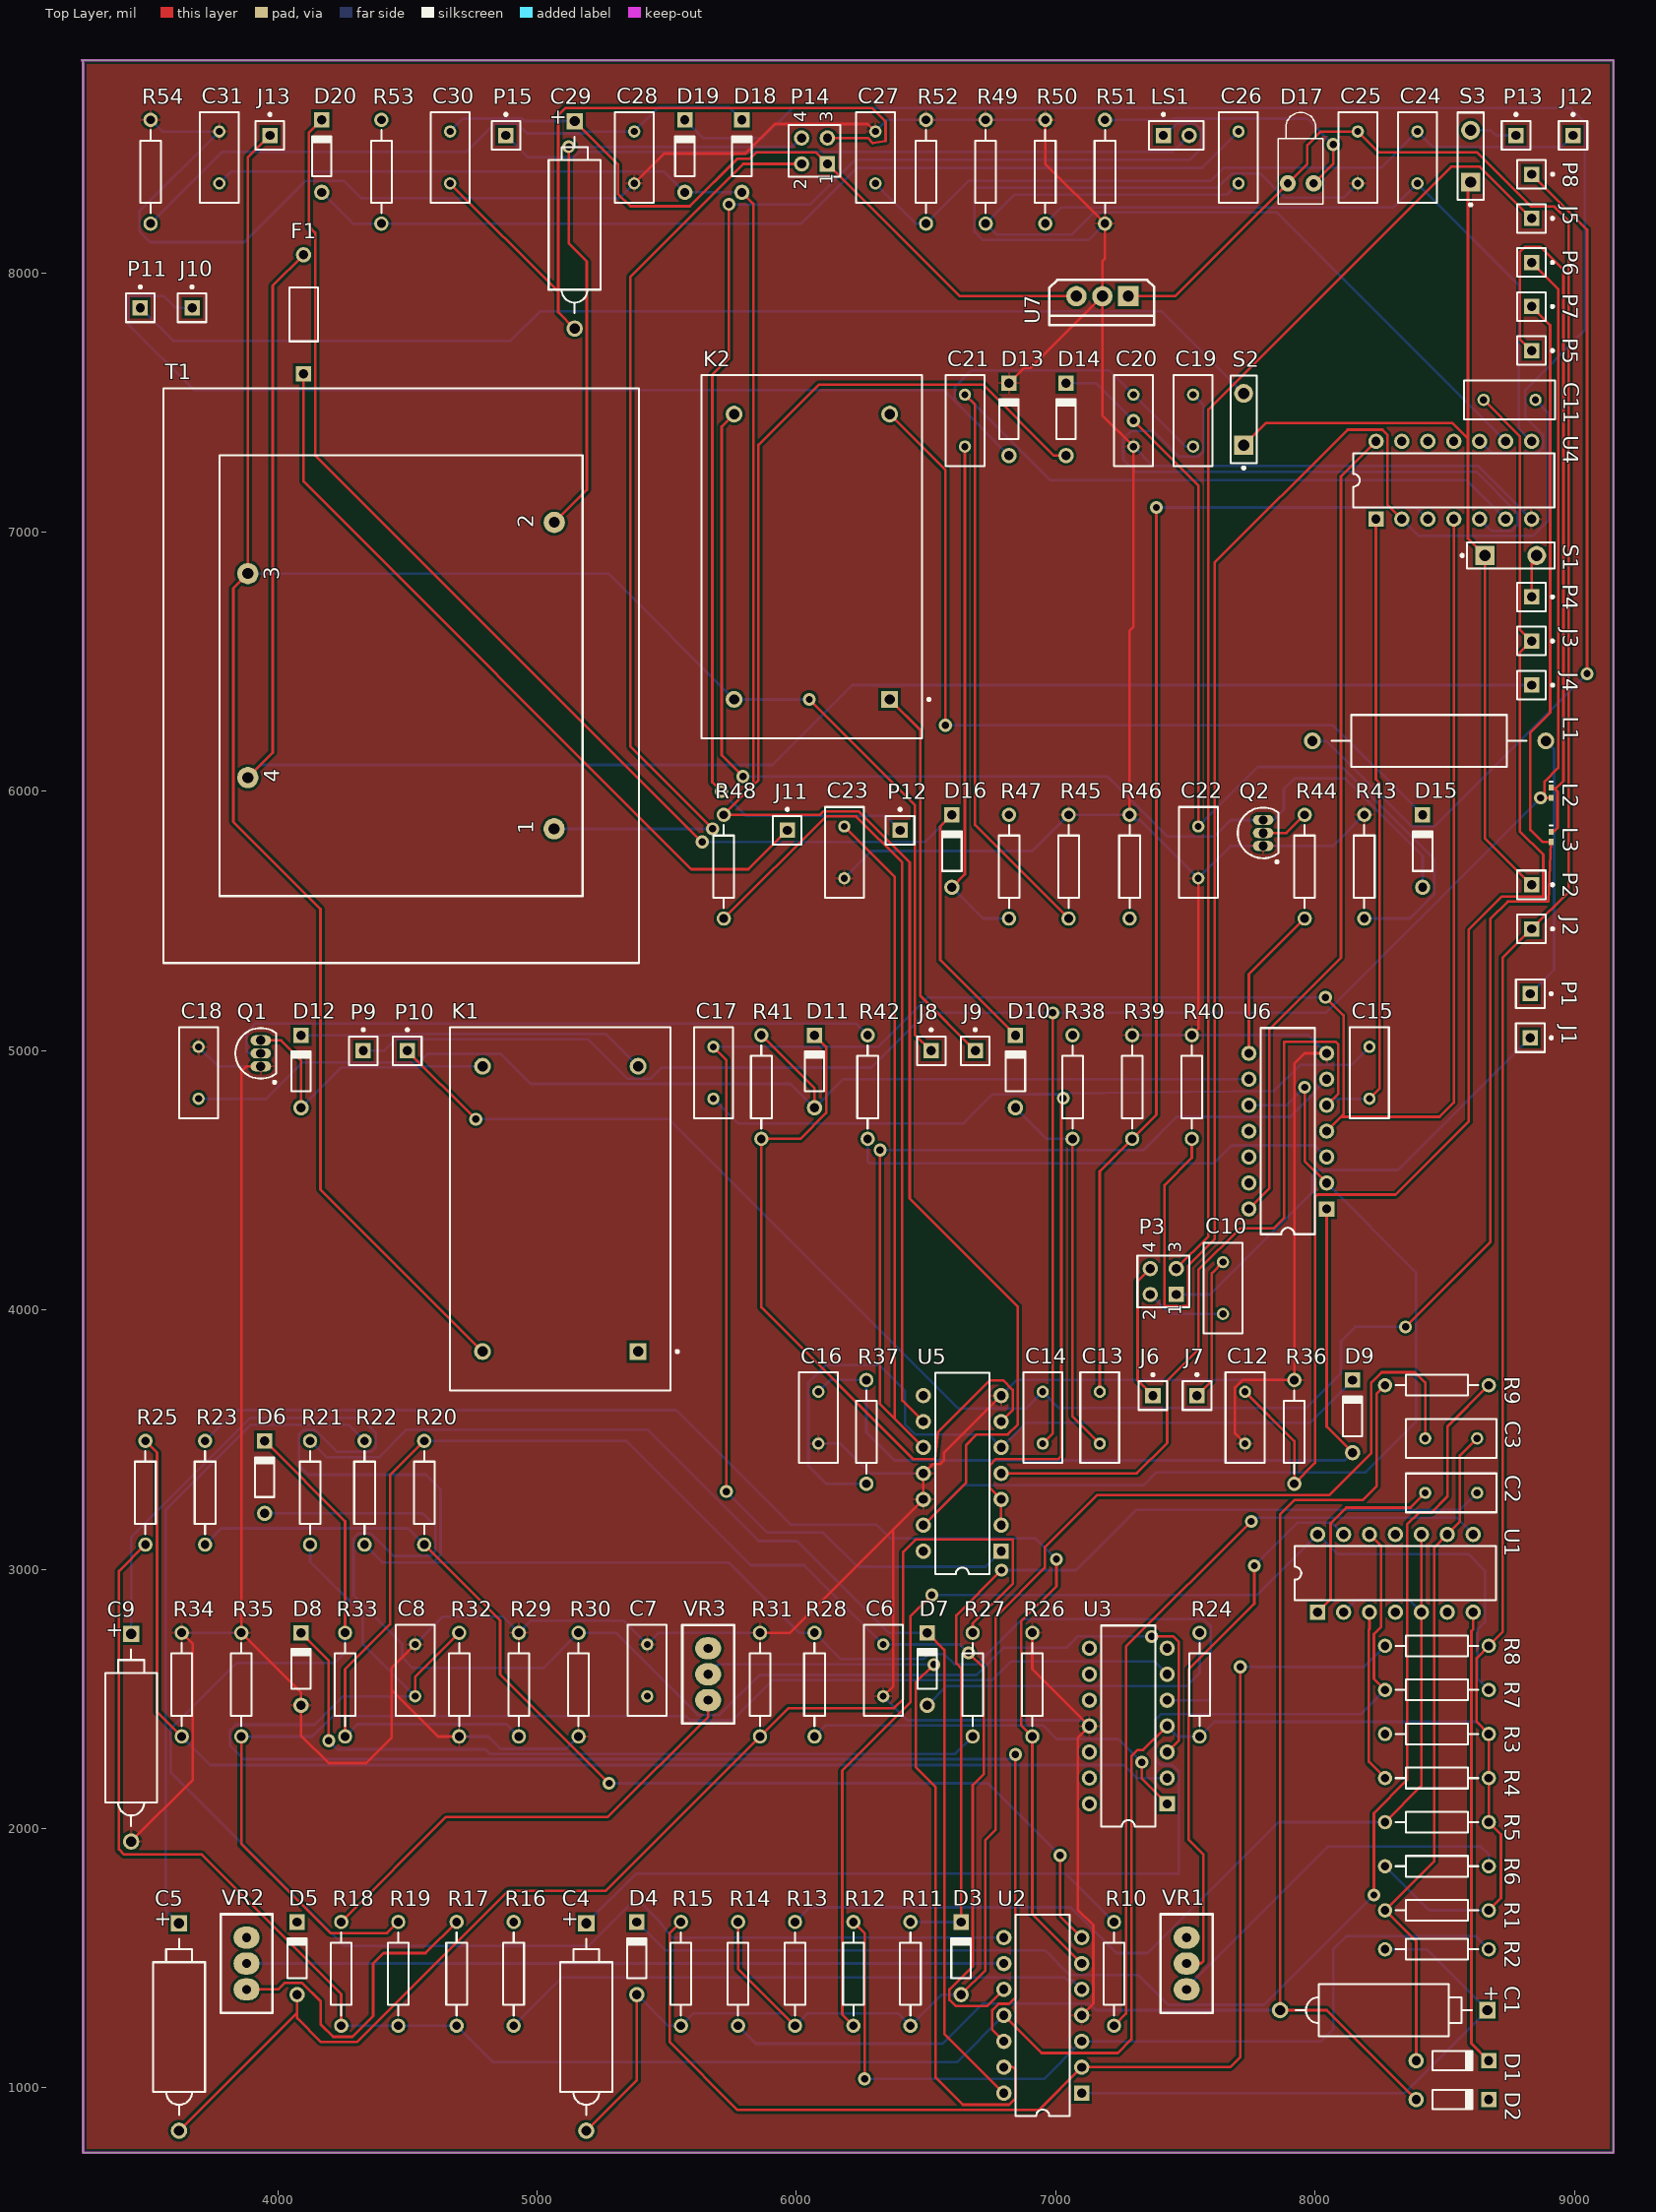
[diagram p0: Top Layer view]
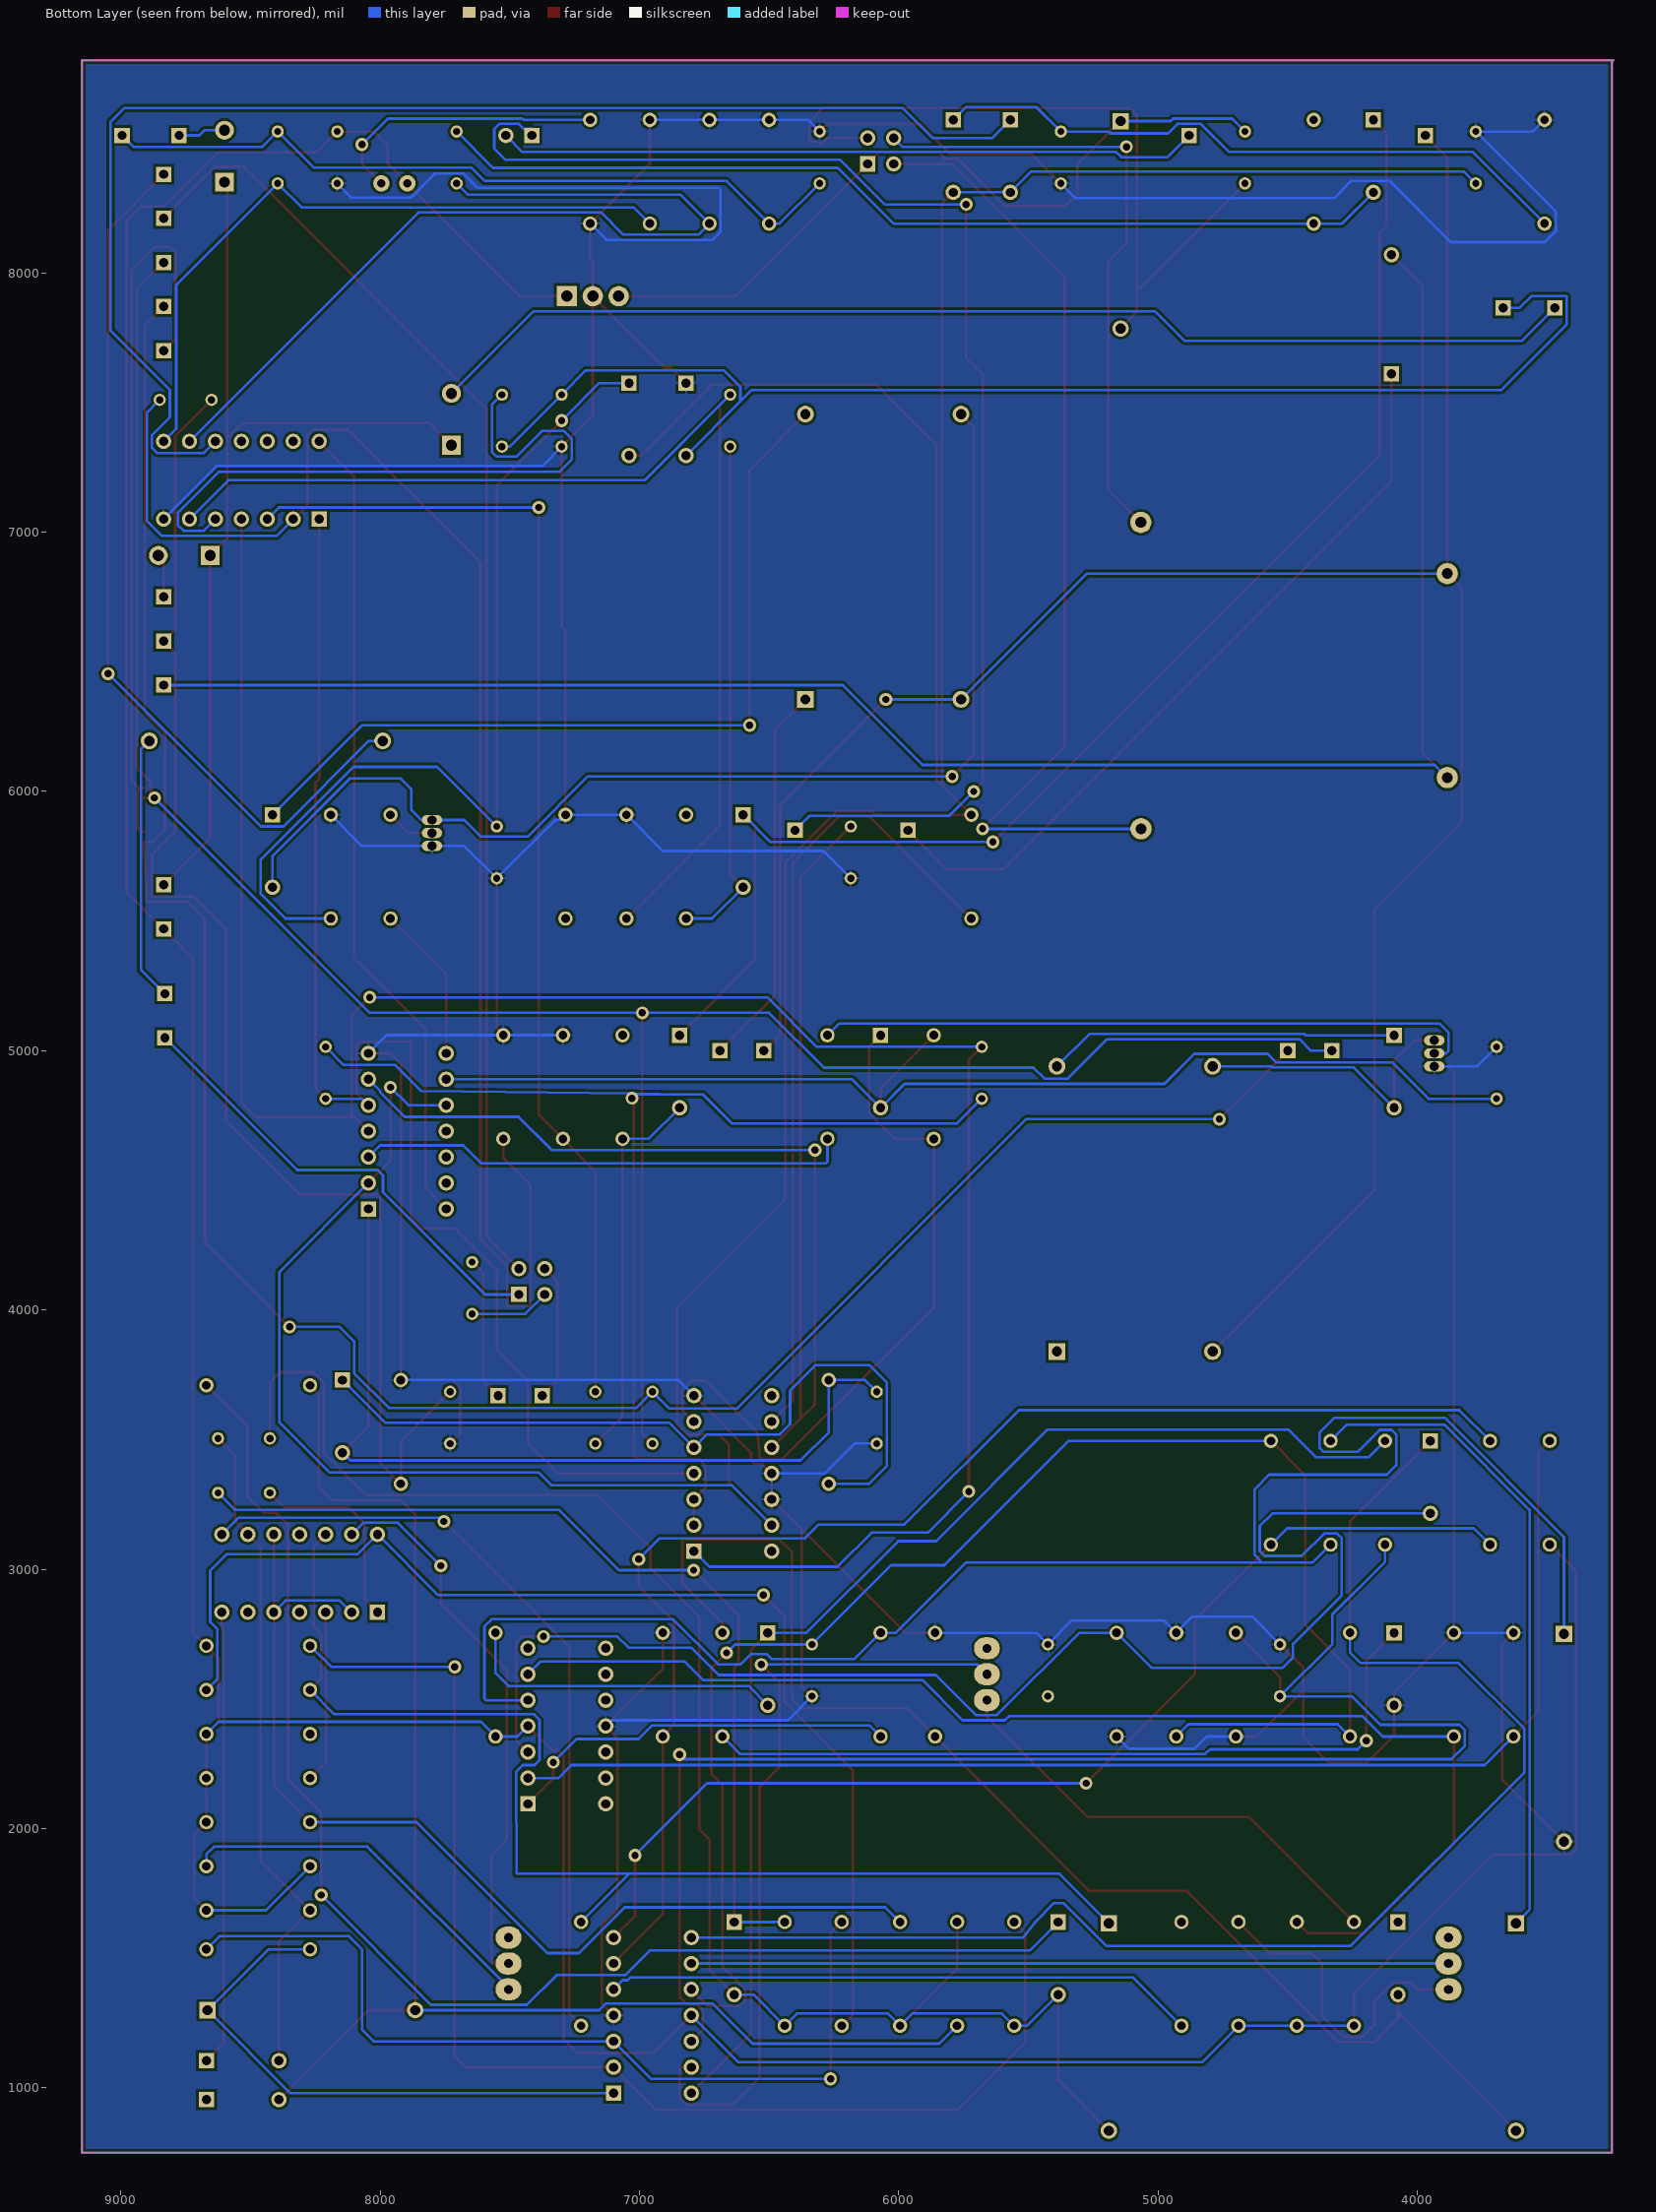
[diagram p1: Bottom Layer view, seen from below]
# Altium PCB MISC82089.PcbDoc (part 1 of 2)
Units mil, origin at the board's own origin, x right, y up, seen from the top; angles counter-clockwise.
Board outline 5905 x 8070 mil, 2 copper layers (Top Layer, Bottom Layer); 156 components, 100 nets, 374 pads, 37 vias.

## Layer stack, top to bottom (the 12.6 mil dielectric is the usual default, probably not edited)
Top Solder: solder mask 0.4, Solder Resist, Dk 3.5
Top Layer: signal copper 1.4
Dielectric 1: dielectric 12.6, FR-4, Dk 4.8
Bottom Layer: signal copper 1.4
Bottom Solder: solder mask 0.4, Solder Resist, Dk 3.5

## Board outline
3250,8750 3250,8807.93 ccw(c3232.93,8807.93) 3245,8820 9150,8820 9150,750 3250,750

## Design rules (kind name [scope] priority, off if disabled: settings)
Clearance [All] p1: gap=10
MinimumSolderMaskSliver [All] p1: minsoldermaskwidth=0
PolygonConnect [All] p1: connectstyle=Relief reliefconductorwidth=10 reliefentries=4 polygonreliefangle="90 Angle" airgapwidth=10
RoutingVias [All] p1: holewidth=28 width=50 viastyle="Through Hole" minholewidth=28 minwidth=50 maxholewidth=28 maxwidth=50
SilkToSilkClearance [All] p1: silktosilkclearance=0
SilkToSolderMaskClearance [IsPad] p1: minsilkscreentomaskgap=0 clearancetoexposedcopper=TRUE
SolderMaskExpansion [All] p1: expansion=4
Width [All] p1: maxlimit=10 minlimit=10 preferedwidth=10
27 further rules are at their usual default settings.

## Components (designator, comment, footprint, x,y, rotation, side; value= is the part's Value field where it differs from the comment)
C1 "220UF" POLAR0.8 8265,1300 r0 top
C2 "0.002" RAD-0.2 8525,3295 r0 top
C3 "104" RAD-0.2 8525,3505 r0 top
C4 "220UF" POLAR0.8 5190,1235 r90 top
C5 "10U" POLAR0.8 3620,1235 r90 top
C6 "104" RAD-0.2 6335,2610.5 r90 top
C7 "105" RAD-0.2 5425,2610.5 r90 top
C8 "105" RAD-0.2 4530,2610.5 r90 top
C9 "220UF" POLAR0.8 3435,2350.5 r90 top
C10 "3.3U" RAD-0.2 7645,4085 r90 top
C11 "105" RAD-0.2 8750,7510 r0 top
C12 "105" RAD-0.2 7730,3585 r90 top
C13 "105" RAD-0.2 7170,3585 r90 top
C14 "3.3U" RAD-0.2 6950,3585 r90 top
C15 "104" RAD-0.2 8210,4915 r90 top
C16 "3.3U" RAD-0.2 6085,3585 r90 top
C17 "104" RAD-0.2 5680,4915 r90 top
C18 "3.3U" RAD-0.2 3695,4915 r90 top
C19 "104" RAD-0.2 7530,7430 r90 top
C20 "104" RAD-0.2 7300,7430 r90 top
C21 "104" RAD-0.2 6650,7430 r90 top
C22 "105" RAD-0.2 7550,5765 r90 top
C23 "104" RAD-0.2 6185,5765 r90 top
C24 "105" RAD-0.2 8395,8445 r90 top
C25 "105" RAD-0.2 8165,8445 r90 top
C26 "105" RAD-0.2 7705,8445 r90 top
C27 "105" RAD-0.2 6305,8445 r90 top
C28 "105" RAD-0.2 5375,8445 r90 top
C29 "220UF" POLAR0.8 5145,8185 r90 top
C30 "105" RAD-0.2 4665,8445 r90 top
C31 "105" RAD-0.2 3775,8445 r90 top
D1 "4148" DO-35 8530,1105 r0 top
D2 "4148" DO-35 8530,955 r0 top
D3 "4148" DO-35 6635,1500 r90 top
D4 "4148" DO-35 5385,1500 r90 top
D5 "4148" DO-35 4075,1500 r90 top
D6 "4148" DO-35 3950,3355.5 r90 top
D7 "4148" DO-35 6505,2615.5 r90 top
D8 "4148" DO-35 4090,2615.5 r90 top
D9 "4148" DO-35 8145,3590 r90 top
D10 "4148" DO-35 6845,4920 r90 top
D11 "4148" DO-35 6070,4920 r90 top
D12 "4148" DO-35 4090,4920 r90 top
D13 "4148" DO-35 6820,7435 r90 top
D14 "4148" DO-35 7040,7435 r90 top
D15 "4148" DO-35 8415,5770 r90 top
D16 "4148" DO-35 6600,5770 r90 top
D17 "LED1" LED-1 7945,8345 r90 top
D18 "4148" DO-35 5790,8450 r90 top
D19 "4148" DO-35 5570,8450 r90 top
D20 "4148" DO-35 4170,8450 r90 top
F1 "Fuse 1" PIN-W2/E2.8 4100,7840 r90 top
J1 "Socket" PIN1 8830,5050 r270 top
J2 "Socket" PIN1 8835,5470 r270 top
J3 "Socket" PIN1 8835,6580 r270 top
J4 "Socket" PIN1 8835,6410 r270 top
J5 "Socket" PIN1 8835,8210 r270 top
J6 "Socket" PIN1 7375,3670 r0 top
J7 "Socket" PIN1 7545,3670 r0 top
J8 "Socket" PIN1 6520,5000 r0 top
J9 "Socket" PIN1 6690,5000 r0 top
J10 "Socket" PIN1 3670,7865 r0 top
J11 "Socket" PIN1 5965,5850 r0 top
J12 "Socket" PIN1 8995,8530 r0 top
J13 "Socket" PIN1 3970,8530 r0 top
K1 "Relay-SPST" MODULE4 5090,4390 r90 top
K2 "Relay-SPST" MODULE4 6060,6905 r90 top
L1 "Inductor Iron" AXIAL-0.9 8440,6195 r0 top
L2 "Inductor" 0402-A 8910,5995 r270 top
L3 "Inductor" 0402-A 8910,5825 r270 top
LS1 "Bell" PIN2 7415,8530 r0 top
P1 "Plug" PIN1 8830,5220 r270 top
P2 "Plug" PIN1 8835,5640 r270 top
P3 "Header 2X2" HDR2X2 7465,4060 r90 top
P4 "Plug" PIN1 8835,6750 r270 top
P5 "Plug" PIN1 8835,7700 r270 top
P6 "Plug" PIN1 8835,8040 r270 top
P7 "Plug" PIN1 8835,7870 r270 top
P8 "Plug" PIN1 8835,8380 r270 top
P9 "Plug" PIN1 4330,5000 r0 top
P10 "Plug" PIN1 4500,5000 r0 top
P11 "Plug" PIN1 3470,7865 r0 top
P12 "Plug" PIN1 6400,5850 r0 top
P13 "Plug" PIN1 8775,8530 r0 top
P14 "Header 2X2" HDR2X2 6120,8420 r90 top
P15 "Plug" PIN1 4880,8530 r0 top
Q1 "2N3904" TO-92A 3935,4990 r0 top
Q2 "2N3904" TO-92A 7800,5840 r0 top
R1 "17" AXIAL-0.4 8470,1685 r0 top
R2 "4" AXIAL-0.4 8470,1535 r0 top
R3 "8" AXIAL-0.4 8470,2365 r0 top
R4 "9" AXIAL-0.4 8470,2195 r0 top
R5 "10" AXIAL-0.4 8470,2025 r0 top
R6 "50" AXIAL-0.4 8470,1855 r0 top
R7 "50" AXIAL-0.4 8470,2535 r0 top
R8 "50" AXIAL-0.4 8470,2705 r0 top
R9 "24" AXIAL-0.4 8470,3710 r0 top
R10 "1.5K" AXIAL-0.4 7225,1440 r90 top
R11 "12" AXIAL-0.4 6440,1440 r90 top
R12 "22" AXIAL-0.4 6220,1440 r90 top
R13 "11" AXIAL-0.4 5995,1440 r90 top
R14 "2" AXIAL-0.4 5775,1440 r90 top
R15 "50" AXIAL-0.4 5555,1440 r90 top
R16 "20K" AXIAL-0.4 4910,1440 r90 top
R17 "50" AXIAL-0.4 4690,1440 r90 top
R18 "10K" AXIAL-0.4 4245,1440 r90 top
R19 "10K" AXIAL-0.4 4465,1440 r90 top
R20 "51" AXIAL-0.4 4565,3295.5 r90 top
R21 "330K" AXIAL-0.4 4125,3295.5 r90 top
R22 "10K" AXIAL-0.4 4335,3295.5 r90 top
R23 "50" AXIAL-0.4 3720,3295.5 r90 top
R24 "10K" AXIAL-0.4 7555,2555.5 r90 top
R25 "10K" AXIAL-0.4 3490,3295.5 r90 top
R26 "49" AXIAL-0.4 6910,2555.5 r90 top
R27 "1K" AXIAL-0.4 6680,2555.5 r90 top
R28 "1K" AXIAL-0.4 6070,2555.5 r90 top
R29 "35" AXIAL-0.4 4930,2555.5 r90 top
R30 "100K" AXIAL-0.4 5160,2555.5 r90 top
R31 "25K" AXIAL-0.4 5860,2555.5 r90 top
R32 "10K" AXIAL-0.4 4700,2555.5 r90 top
R33 "28" AXIAL-0.4 4260,2555.5 r90 top
R34 "3M" AXIAL-0.4 3630,2555.5 r90 top
R35 "10K" AXIAL-0.4 3860,2555.5 r90 top
R36 "49" AXIAL-0.4 7920,3530 r90 top
R37 "510K" AXIAL-0.4 6270,3530 r90 top
R38 "5.1K" AXIAL-0.4 7065,4860 r90 top
R39 "5.1K" AXIAL-0.4 7295,4860 r90 top
R40 "5.1K" AXIAL-0.4 7525,4860 r90 top
R41 "510K" AXIAL-0.4 5865,4860 r90 top
R42 "1K" AXIAL-0.4 6275,4860 r90 top
R43 "51K" AXIAL-0.4 8190,5710 r90 top
R44 "1K" AXIAL-0.4 7960,5710 r90 top
R45 "5.1K" AXIAL-0.4 7050,5710 r90 top
R46 "5.1K" AXIAL-0.4 7285,5710 r90 top
R47 "5.1K" AXIAL-0.4 6820,5710 r90 top
R48 "10K" AXIAL-0.4 5720,5710 r90 top
R49 "51K" AXIAL-0.4 6730,8390 r90 top
R50 "51K" AXIAL-0.4 6960,8390 r90 top
R51 "15K" AXIAL-0.4 7190,8390 r90 top
R52 "51K" AXIAL-0.4 6500,8390 r90 top
R53 "51K" AXIAL-0.4 4400,8390 r90 top
R54 "51K" AXIAL-0.4 3510,8390 r90 top
S1 "SW-PB" SPST-2 8755,6910 r0 top
S2 "SW-PB" SPST-2 7725,7435 r90 top
S3 "SW-PB" SPST-2 8600,8450 r90 top
T1 "Trans Eq" TRF_4 4475.83,6446.67 r90 top
U1 "LM324N" 646-06 8310,2985 r0 top
U2 "LM324N" 646-06 6950,1280 r90 top
U3 "LM324N" 646-06 7280,2395.5 r90 top
U4 "SN74LS02N" N014 8535,7200 r0 top
U5 "SN74LS74AN" 646-06 6640,3370 r90 top
U6 "SN74LS08J" J014 7895,4690 r90 top
U7 "LM7805" TO220A 7180,7910 r180 top
VR1 "10K" 3296W 7505,1480 r90 top
VR2 "10K" 3296W 3880,1480 r90 top
VR3 "10K" 3296W 5660,2595.5 r90 top

## Footprints (in the part's own frame and the unit in brackets; to place one, negate y for a bottom-side part, rotate by r counter-clockwise, add the part's x,y. Pads: shape width x height; smd on the part's side, far side on the other; paste and mask are expansions set on the pad)
0402-A [mm] "Chip Inductor, Body 1.0x0.5mm, IPC High Density"
  rect 0.6x0.5 smd: 1(-0.5,0) 2(0.5,0)
  silkscreen extent -1.1,-0.15 -1.1,0.15, body extent -0.55,-0.3 0.55,0.3, height 0.55
646-06 [mm] "DIP; 14 Leads; Row Spacing 7.62 mm; Pitch 2.54 mm"
  rect 1.5x1.5 hole 0.9: 1(-7.62,-3.81)
  round 1.5 hole 0.9: 2(-5.08,-3.81) 3(-2.54,-3.81) 4(0,-3.81) 5(2.54,-3.81) 6(5.08,-3.81) 7(7.62,-3.81) 8(7.62,3.81) 9(5.08,3.81) 10(2.54,3.81) 11(0,3.81) 12(-2.54,3.81) 13(-5.08,3.81) 14(-7.62,3.81)
  silkscreen extent -9.85,-2.65 9.85,2.65
3296W [mil]
  oval 85x100 hole 35: 1(-100,0) 2(0,0) 3(100,0)
  silkscreen extent -190,-100 190,100, body extent -188,-94 188,94, height 455
AXIAL-0.4 [mm] "Axial Device, Thru-Hole; 2 Leads; 0.4 in Pin Spacing"
  round 1.4 hole 0.85: 1(-5.08,0) 2(5.08,0)
  silkscreen extent -4.06,-1.02 4.06,1.02
AXIAL-0.9 [mm] "Axial Device, Thru-Hole; 2 Leads; 0.9 in Pin Spacing"
  round 1.65 hole 1: 1(-11.43,0) 2(11.43,0)
  silkscreen extent -9.53,-2.54 9.53,2.54
DO-35 [mm] "Diode, Axial; Body 3.8 x 1.9 mm (LxDia. max), Lead Dia. 0.53 mm (max)"
  round 1.5 hole 0.9: 1(-3.55,0)
  rect 1.5x1.5 hole 0.9: 2(3.55,0)
  silkscreen extent -1.95,-0.95 2.05,0.95
HDR2X2 [mm] "Connector; Header; 2x2 Position"
  rect 1.5x1.5 hole 0.9: 1(0,0)
  round 1.5 hole 0.9: 2(0,2.54) 3(2.54,0) 4(2.54,2.54)
  silkscreen extent -1.27,-1.27 3.81,3.81
J014 [mm] "DIP; 14 Leads; Row Spacing 7.62 mm; Pitch 2.54 mm"
  rect 1.5x1.5 hole 0.9: 1(-7.62,-3.81)
  round 1.5 hole 0.9: 2(-5.08,-3.81) 3(-2.54,-3.81) 4(0,-3.81) 5(2.54,-3.81) 6(5.08,-3.81) 7(7.62,-3.81) 8(7.62,3.81) 9(5.08,3.81) 10(2.54,3.81) 11(0,3.81) 12(-2.54,3.81) 13(-5.08,3.81) 14(-7.62,3.81)
  silkscreen extent -10.1,-2.65 10.1,2.65
LED-1 [mm] "LED; 2 Leads"
  round 1.6 hole 0.8: 1(0,1.27) 2(0,-1.27)
  silkscreen extent -2,-2.2 6.95,2.2
MODULE4 [mm] "DIP; 4 Round Pins; Row Space 27.94 mm; Pitch 15.24 mm"
  rect 1.65x1.65 hole 1: 1(-13.97,-7.62)
  round 1.65 hole 1: 2(-13.97,7.62) 3(13.97,-7.62) 4(13.97,7.62)
  silkscreen extent -17.8,-11.58 17.8,10.8, body extent -17.8,-10.8 17.8,10.8, height 14
N014 [mm] "DIP; 14 Leads; Row Spacing 7.62 mm; Pitch 2.54 mm"
  rect 1.5x1.5 hole 0.9: 1(-7.62,-3.81)
  round 1.5 hole 0.9: 2(-5.08,-3.81) 3(-2.54,-3.81) 4(0,-3.81) 5(2.54,-3.81) 6(5.08,-3.81) 7(7.62,-3.81) 8(7.62,3.81) 9(5.08,3.81) 10(2.54,3.81) 11(0,3.81) 12(-2.54,3.81) 13(-5.08,3.81) 14(-7.62,3.81)
  silkscreen extent -9.85,-2.65 9.85,2.65
PIN1 [mm] "Connector; Plug"
  rect 1.5x1.5 hole 0.9: 1(0,0)
  silkscreen extent -1.4,-1.4 1.4,2.18
PIN2 [mm] "Photosensitive Diode; 2 Leads"
  rect 1.5x1.5 hole 0.9: 1(0,0)
  round 1.5 hole 0.9: 2(2.54,0)
  silkscreen extent -1.4,-1.4 3.94,2.17
PIN-W2/E2.8 [mm] "Thru-Hole; 2 Leads"
  rect 1.5x1.5 hole 0.9: 1(-5.825,0)
  round 1.5 hole 0.9: 2(5.825,0)
  silkscreen extent -2.65,-1.4 2.65,1.4
POLAR0.8 [mm] "Polarized Capacitor; 2 Leads"
  rect 1.6x1.6 hole 1: 1(10.16,0)
  round 1.6 hole 1: 2(-10.16,0)
  silkscreen extent -8.64,-2.54 8.64,2.54
RAD-0.2 [mm] "Radial Cap, Thru-Hole; 2 Leads; 0.2 in Pin Spacing"
  round 1.2 hole 0.7: 1(-2.54,0) 2(2.54,0)
  silkscreen extent -4.44,-1.91 4.44,1.91
SPST-2 [mm] "Switch; 2 Leads"
  rect 1.85x1.85 hole 1.1: 1(-2.54,0)
  round 1.85 hole 1.1: 2(2.54,0)
  silkscreen extent -4.89,-1.27 4.28,1.27
TO220A [mm] "220，3脚晶体管"
  rect 2x2 hole 1.1: 1(-2.54,0)
  round 2 hole 1.1: 2(0,0) 3(2.54,0)
  silkscreen extent -5.08,-1.6 5.21,2.82, body extent -5.08,-1.45 5.22,2.98, height 18.5
TO-92A [mm] "TO, Flat Index; 3 In-Line, Axial Leads; Body Dia. 4.5mm; Leads 0.51 x 0.48 mm (max)"
  oval 2x1 hole 0.9: 1(0,-1.27) 2(0,0) 3(0,1.27)
  silkscreen extent -2.48,-2.95 1.5,2.48, body extent -2.48,-2.5 1.5,2.5, height 6.86
TRF_4 [mil] "Transformer; 4 Leads"
  round 82 hole 42: 1(-590.83,-590) 2(590.83,-590.83) 3(393.33,590.83) 4(-393.33,590.83)
  silkscreen extent -1108,-917 1108,917

## Part data
C1 C4 C5 C9 C29: library part "Cap Pol2", "Polarized Capacitor (Axial)"
C2 C3 C6 C7 C8 C10 C11 C12 C13 C14 C15 C16 C17 C18 C19 C20 C21 C22 C23 C24 C25 C26 C27 C28 C30 C31: library part Cap, "Capacitor"
D1 D2 D3 D4 D5 D6 D7 D8 D9 D10 D11 D12 D13 D14 D15 D16 D18 D19 D20: library part "Diode 1N914", "High Conductance Fast Diode"
D17: "Typical RED GaAs LED"
F1: "Fuse"
K1 K2: "Single-Pole Single-Throw Relay"
L1: "Magnetic-Core Inductor"
LS1: "Electrical Bell"
P3 P14: "Header, 2-Pin, Dual row"
Q1 Q2: "NPN General Purpose Amplifier"
R1 R2 R3 R4 R5 R6 R7 R8 R9 R10 R11 R12 R13 R14 R15 R16 R17 R18 R19 R20 R21 R22 R23 R24 R25 R26 R27 R28 R29 R30 R31 R32 R33 R34 R35 R36 R37 R38 R39 R40 R41 R42 R43 R44 R45 R46 R47 R48 R49 R50 R51 R52 R53 R54: library part Res2, "Resistor"
S1 S2 S3: "Switch"
T1: "Transformer (Equivalent Circuit Model)"
U1 U2 U3: "Quad Low-Power Operational Amplifier"
U4: "Quadruple 2-Input Positive-NOR Gate"
U5: "Dual D-Type Positive Edge-Triggered Flip-Flop"
U6: "Quadruple 2-Input Positive-AND Gate"
VR1 VR2 VR3: library part RESVR

## Via types
v1: diameter 50, hole 28, Top Layer to Bottom Layer, 37 vias

## Nets (pads, with @x,y where several pads share a name; then routed paths per layer and width w, separated by ;. In a path a pad name is that pad's centre, name@x,y a point inside that pad or via, vN(x,y) a via of type N, cw(c..) or ccw(c..) an arc to the next point about the centre after c; other vN are vias at no path point)
+5: C25.2 D17.1 J2.1 R1.2 R3.2 R4.2 R5.2 R6.1 R8.2 R17.1 R18.1 R19.1 R24.1 R25.1 U2.11 U3.4 U7.1 | length 17604.8
  Top Layer w10: R25.1@3490,3095.5 3388,2993.5 3388,1920 3408,1900 3707.52,1900 4245,1362.52 R18.1@4245,1240 ; U2.11@6800,1280 6945,1135 7240,1135 7292,1187 7292,2280 7315.22,2303.22 7337.73,2303.22 U3.4@7430,2395.5 ; U7.1@7280,7910 7460,7910 D17.1@7895,8345 7970.61,8420.61 7970.61,8492.51 8023.1,8545 C25.2@8165,8545 8245,8465 8623,8465 8832,8256 8921,8256 8978,8199 8978,5613 J2.1@8835,5470 8723,5358 8723,2758 R8.2@8670,2705 8623,2658 8623,2412 R3.2@8670,2365 R4.2@8670,2195 R5.2@8670,2025 8717,1978 8717,1732 R1.2@8670,1685
  Bottom Layer w10: R18.1@4245,1240 R19.1@4465,1240 R17.1@4690,1240 4831,1099 6619,1099 U2.11@6800,1280 ; U3.4@7430,2395.5 7470,2355.5 R24.1@7555,2355.5 7611.5,2412 8623,2412 R3.2@8670,2365 ; R6.1@8270,1855 8440,1685 R1.2@8670,1685
GND: C6.1 C7.2 C8.2 C9.2 C12.1 C16.1 C18.2 C20.1 C22.1 C23.1 C25.1 C27.2 C28.1 C31.2 D8.1 D13.2 Q1.1 Q2.1 R26.2 R29.2 R30.1 R31.2 R32.1 R34.2 R35.2 R36.2 R39.2 R40.2 R43.2 R45.2 R46.2 R49.2 R50.2 R51.1 R52.2 R54.2 U2.4 U3.11 U4.7 U5.7 U5.11 U5.12 U6.7 U7.2 | length 30799.8
  Top Layer w10: C9.2@3435,1950.5 3673,2188.5 3673,2712.5 R34.2@3630,2755.5 ; Q1.1@3935,4940 3880,4940 3860,4920 R35.2@3860,2755.5 4090,2525.5 D8.1@4090,2475.73 4090,2360 4197.06,2252.94 4340.94,2252.94 4440,2352 4440,2534.5 ; C8.2@4530,2710.5 4440,2620.5 4440,2534.5 ; R32.1@4700,2355.5 4619,2355.5 4440,2534.5 ; C28.1@5375,8345 5490,8460 5804,8460 5918,8574 6276,8574 C27.2@6305,8545 ; R31.2@5860,2755.5 5975.5,2755.5 6374,3154 ; C6.1@6335,2510.5 6374,2549.5 6374,3154 ; U5.7@6790,3670 6568.84,3448.84 6568.84,3420 6554.32,3405.47 6525.47,3405.47 U5.11@6490,3370 U5.12@6490,3270 6374,3154 ; D13.2@6820,7574.76 6879.24,7634 6904,7634 U7.2@7180,7910 ; R26.2@6910,2755.5 6910,2615.5 U3.11@7130,2395.5 7085,2350.5 7085,1688 7145,1628 7145,1325 U2.4@7100,1280 ; R50.2@6960,8590 6960,8420 R51.1@7190,8190 7190,8055 7180,8045 U7.2@7180,7910 ; R46.2@7285,5910 7285,6620 7300,6635 C20.1@7300,7330 7180,7450 U7.2@7180,7910 ; R40.2@7525,5060 7550,5085 C22.1@7550,5665 ; C12.1@7730,3485 7691,3524 7691,3701 7720,3730 R36.2@7920,3730 7920,4950 7960,4990 U6.7@8045,4990
  Bottom Layer w10: R54.2@3510,8590 3555,8545 C31.2@3775,8545 3467,8237 3467,8160 3509,8118 3871,8118 4108,8355 4255,8355 4322,8288 5318,8288 C28.1@5375,8345 ; R34.2@3630,2755.5 R35.2@3860,2755.5 ; C18.2@3695,5015 3770,4940 Q1.1@3935,4940 ; C8.2@4530,2710.5 4637.56,2818.06 4867.44,2818.06 R29.2@4930,2755.5 4977.5,2803 5332.5,2803 C7.2@5425,2710.5 5470,2755.5 R31.2@5860,2755.5 ; R32.1@4700,2355.5 4812.57,2355.5 4860.07,2308 5112.5,2308 R30.1@5160,2355.5 ; C16.1@6085,3485 6170,3485 6285,3370 U5.11@6490,3370 ; C23.1@6185,5665 6290,5770 6910,5770 R45.2@7050,5910 R46.2@7285,5910 7305,5890 7325,5890 C22.1@7550,5665 7675,5790 Q2.1@7800,5790 8070,5790 R43.2@8190,5910 ; C27.2@6305,8545 6350,8590 R52.2@6500,8590 R49.2@6730,8590 R50.2@6960,8590 ; C6.1@6335,2510.5 6427.44,2418.06 7107.44,2418.06 U3.11@7130,2395.5 ; U5.7@6790,3670 6850,3730 R36.2@7920,3730 ; R51.1@7190,8190 7127.44,8127.44 6717.56,8127.44 6687,8158 6687,8319 6696,8328 7624.38,8328 7680,8383.62 7788,8383.62 7881.62,8290 8110,8290 C25.1@8165,8345 ; R39.2@7295,5060 R40.2@7525,5060 7975,5060 U6.7@8045,4990 ; C20.1@7300,7330 7374.62,7255.38 8629.62,7255.38 U4.7@8835,7050
NetC1_1: C1.1 R2.1 U2.1 | length 2189.9
  Bottom Layer w10: U2.1@7100,980 8345,980 C1.1@8665,1300 8430,1535 R2.1@8270,1535
NetC1_2: C1.2 D2.1 R9.1 R14.1 | length 5593.3
  Top Layer w10: R9.1@8270,3710 8237,3677 8237,3320 8184,3267 7920,3267 7865,3212 C1.2@7865,1300 8045.24,1300 D2.1@8390.24,955
  Bottom Layer w10: R14.1@5775,1240 5844,1171 6564,1171 6718,1325 7130,1325 7155,1300 C1.2@7865,1300
NetC2_1: C2.1 U1.1 | length 777.2
  Top Layer w10: U1.1@8010,2835 8060,2885 8060,3178 8120,3238 8368,3238 C2.1@8425,3295
NetC2_2: C2.2 D3.2 R11.2 | length 3589.3
  Top Layer w10: D3.2@6635,1639.76 6635,2620 6617,2638 6617,2823 v1(6791,2997)
  Bottom Layer w10: R11.2@6440,1640 6479.52,1640 6479.76,1639.76 D3.2@6635,1639.76 ; v1(6791,2997) 7079,2997 7312,3230 8560,3230 C2.2@8625,3295
NetC3_1: C3.1 C4.2 D3.1 D4.1 R11.1 R13.1 R14.2 R15.1 | length 6520.4
  Top Layer w10: C4.2@5190,835 5385,1030 D4.1@5385,1360.24 ; R14.2@5775,1640 5775,1460 R13.1@5995,1240 ; D3.1@6635,1360.24 6729,1454.24 6729,1956 6769,1996 6769,2817.37 6957.88,3006.25 6957.88,3084.5 7160.38,3287 8056,3287 8217,3448 8217,3720 8257,3760 8385,3760 8425,3720 C3.1@8425,3505
  Bottom Layer w10: D4.1@5385,1360.24 5505.24,1240 R15.1@5555,1240 5602,1287 5948,1287 R13.1@5995,1240 6042,1287 6393,1287 R11.1@6440,1240 6560.24,1360.24 D3.1@6635,1360.24
NetC3_2: C3.2 D1.1 R1.1 U1.9 | length 2596.8
  Top Layer w10: D1.1@8390.24,1105 8390.24,1564.76 R1.1@8270,1685 8460,1875 8460,3085 U1.9@8510,3135 8559,3184 8559,3439 C3.2@8625,3505
NetC4_1: C4.1 R7.1 R10.2 U1.12 | length 4864.1
  Top Layer w10: U1.12@8210,3135 8255,3090 8255,2778 8227.44,2750.44 8227.44,2577.56 R7.1@8270,2535
  Bottom Layer w10: C4.1@5190,1635 5381,1826 7039,1826 ; R10.2@7225,1640 7039,1826 ; R7.1@8270,2535 8176,2441 7406,2441 7385,2420 7385,2265 7405,2245 7450,2245 7475,2220 7474,1826 7039,1826
NetC5_1: C5.1 R22.2 | length 2545.2
  Bottom Layer w10: C5.1@3620,1635 3567.44,1687.56 3567.44,3228.44 3897.06,3558.06 4272.44,3558.06 R22.2@4335,3495.5
NetC5_2: C5.2 D5.1 R27.2 R31.1 | length 5091
  Top Layer w10: C5.2@3620,835 4075,1290 ; D5.1@4075,1360.24 4075,1290 ; R27.2@6680,2755.5 6680,2791 6835,2946 6835,3115 6460,3115 6412.06,3067.06 6412.06,2500.06 6377,2465 5969.5,2465 R31.1@5860,2355.5 5264.5,1760 4889,1760 4306.44,1177.44 4166.56,1177.44 4075,1269 4075,1290
NetC6_2: C6.2 R20.2 R29.1 R33.1 U2.10 | length 6076.9
  Top Layer w10: R33.1@4260,2355.5 4260,2615 4433,2788 4433,3363.5 R20.2@4565,3495.5 ; v1(6664,2678) 6723,2619 6723,2211 6680,2168 6680,1469.53 6590.47,1380 6590.47,1340 6614.76,1315.71 6735.71,1315.71 U2.10@6800,1380
  Bottom Layer w10: R33.1@4260,2355.5 4307.5,2403 4882.5,2403 R29.1@4930,2355.5 ; R20.2@4565,3495.5 5344.5,3495.5 5824,3016 6029.5,3016 C6.2@6335,2710.5 6631.5,2710.5 v1(6664,2678)
NetC8_1: C8.1 R21.1 R32.2 U2.12 | length 6137.2
  Top Layer w10: C8.1@4530,2510.5 4530,2585.5 R32.2@4700,2755.5 ; U2.12@6800,1180 6755.47,1224.53 6755.47,1300 6780,1324.53 6820,1324.53 6845,1349.53 v1(6845,2286)
  Bottom Layer w10: R21.1@4125,3095.5 4125,3030 4328,2827 4328,2712.5 C8.1@4530,2510.5 4252.5,2510.5 4143,2401 3838,2401 3817,2380 3817,2320 3869,2268 6827,2268 v1(6845,2286)
NetC9_1: C9.1 R22.1 R28.2 U3.5 | length 6934.2
  Bottom Layer w10: C9.1@3435,2750.5 3435,3125 3895,3585 4320,3585 4378,3527 4378,3470 4360.94,3452.94 4230.06,3452.94 4144.94,3538.06 4100,3538.06 4082,3520.06 4082,3401 4118,3365 4572,3365 4628,3309 4628,3055 4600,3027 ; R22.1@4335,3095.5 4403.5,3027 4600,3027 ; U3.5@7430,2495.5 7592,2495.5 7598,2501.5 7598,2780 7570,2808 6870.44,2808 6696.44,2634 6609.47,2634 6570.47,2673 6509,2673 6490,2654 6171.5,2654 R28.2@6070,2755.5 6011.06,2755.5 5739.56,3027 4600,3027
NetC10_1: C10.1 P3.2 | length 311.1
  Bottom Layer w10: P3.2@7365,4060 7440,3985 C10.1@7645,3985
NetC10_2: C10.2 J7.1 | length 556.4
  Top Layer w10: J7.1@7545,3670 7602,3727 7602,4142 C10.2@7645,4185
NetC11_1: C11.1 C12.2 J3.1 R36.1 | length 5413.4
  Top Layer w10: C12.2@7730,3685 7920,3495 R36.1@7920,3330 8000,3410 8000,4435 8010,4445 8310,4445 8593,4728 8593,5468 8720,5595 8880,5595 8880,5757 8790,5847 8790,6535 J3.1@8835,6580 8790,6625 8790,7370 C11.1@8650,7510
NetC11_2: C11.2 R40.1 U4.2 | length 6025.4
  Top Layer w10: R40.1@7525,4660 7525,4587 7420,4482 7420,4015 7510,4015 7510,4169.99 7613,4272.99 7613,6882 8126,7395 8260,7395 8280,7375 8280,7105 U4.2@8335,7050
  Bottom Layer w10: U4.2@8335,7050 8399.53,6985.47 8840.47,6985.47 8899.53,7044.53 8899.53,7460.47 C11.2@8850,7510
NetC13_1: C13.1 D10.1 R38.1 | length 1488.3
  Top Layer w10: R38.1@7065,4660 7065,3590 C13.1@7170,3485
  Bottom Layer w10: D10.1@6845,4780.24 6965.24,4660 R38.1@7065,4660
NetC13_2: C13.2 R39.1 U4.3 | length 4565.9
  Top Layer w10: C13.2@7170,3685 7170,4535 R39.1@7295,4660 7388,4753 v1(7388,7095)
  Bottom Layer w10: v1(7388,7095) 8390,7095 U4.3@8435,7050